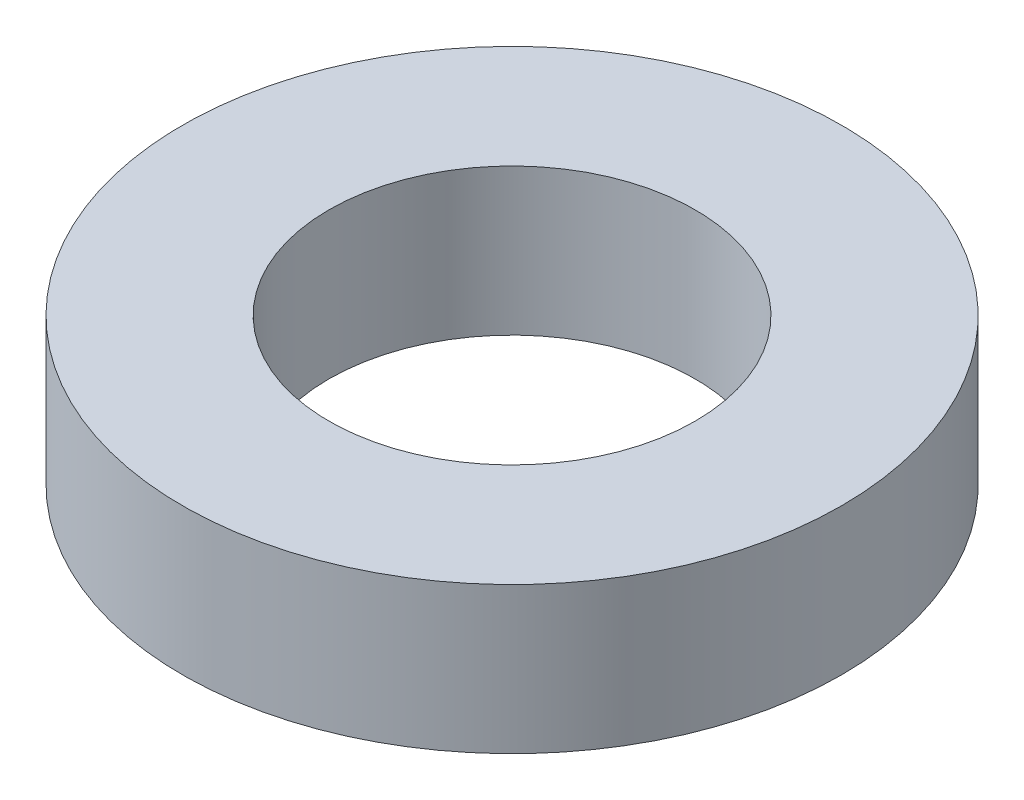
from build123d import *

# Parameters (mm, degrees)
SKETCH1_W = 4
SKETCH1_H = 4


with BuildPart() as part:
    # Sketch1 → Revolve1 (revolve)
    with BuildSketch(Plane.XY):
        with Locations((7, -2)):
            Rectangle(SKETCH1_W, SKETCH1_H)
    revolve(axis=Axis((0, -473.381125867, 0), (0, 1, 0)))


solid = part.part
